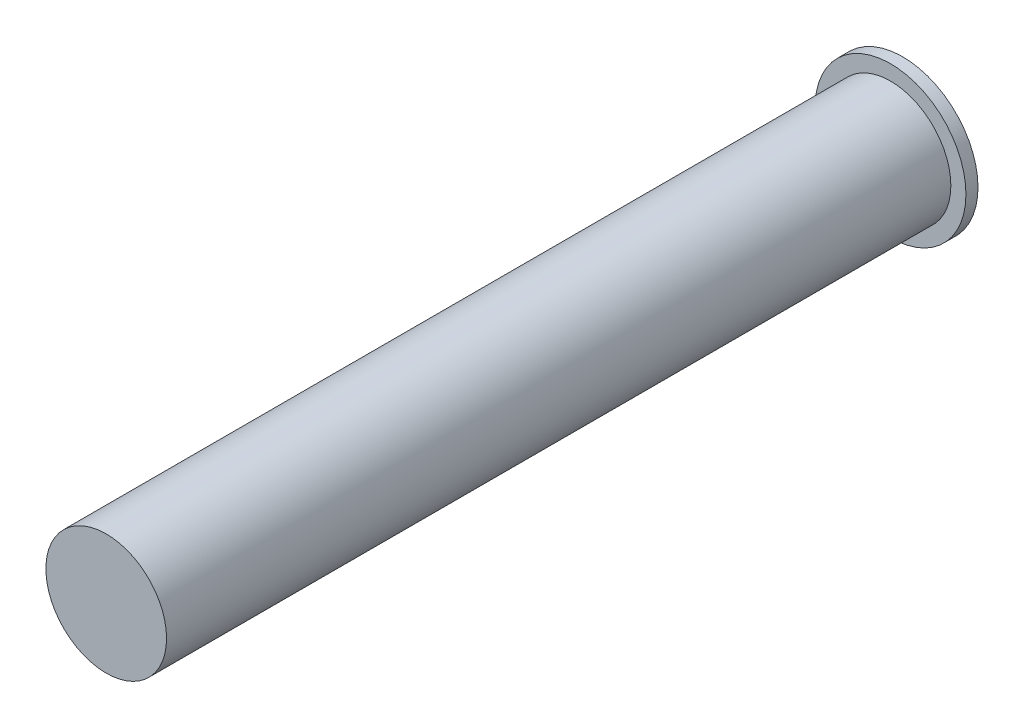
from build123d import *

# Parameters (mm, degrees)
SKETCH1_R           = 12.5
BOSS_EXTRUDE1_DEPTH = 2
SKETCH2_R           = 10
BOSS_EXTRUDE7_DEPTH = 130


with BuildPart() as part:
    # Sketch1 → Boss-Extrude1 (new body)
    with BuildSketch(Plane.XY):
        Circle(SKETCH1_R)
    extrude(amount=BOSS_EXTRUDE1_DEPTH)

    # Sketch2 → Boss-Extrude7 (add)
    with BuildSketch(Plane.XY.offset(2)):
        Circle(SKETCH2_R)
    extrude(amount=BOSS_EXTRUDE7_DEPTH)


solid = part.part
